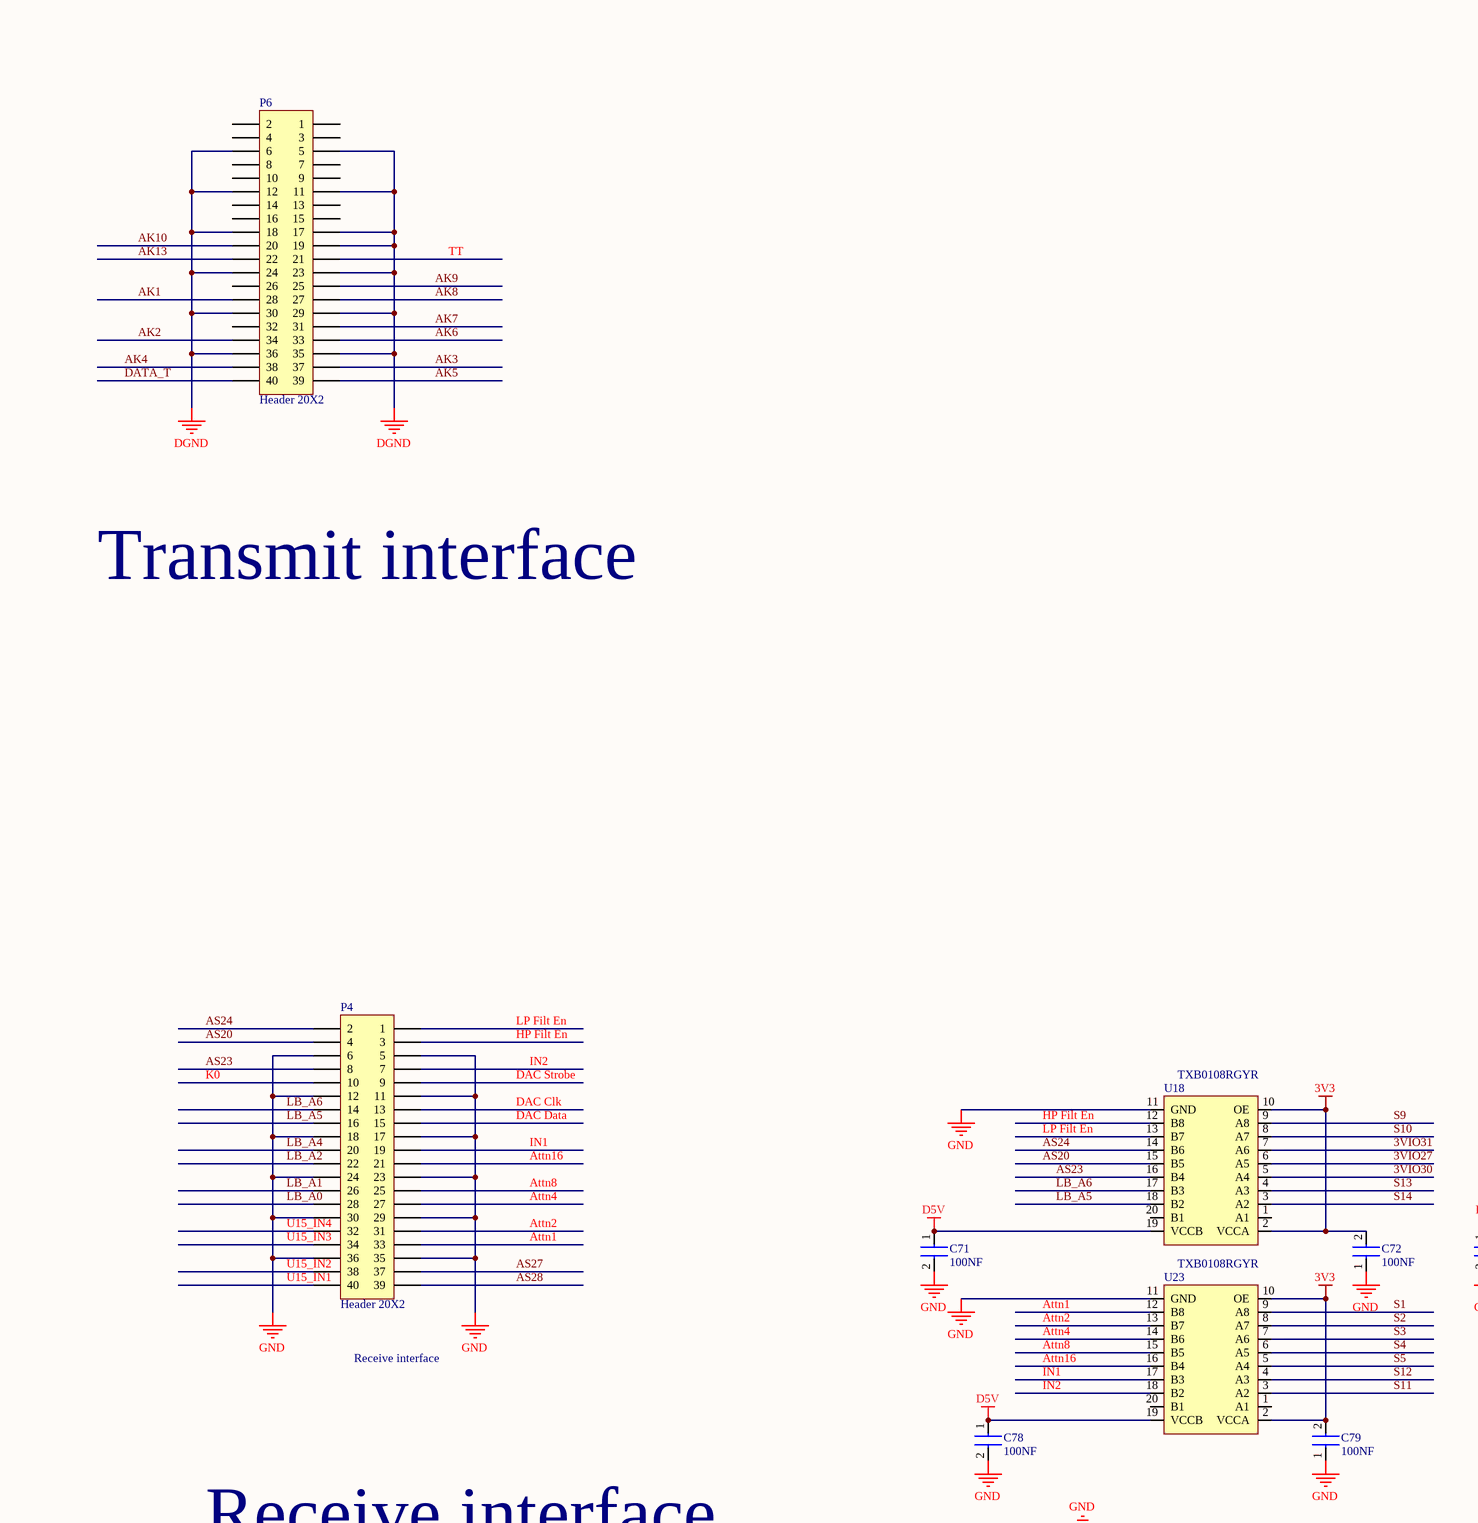
[diagram p0: MISC82191-3.SchDoc, top left]
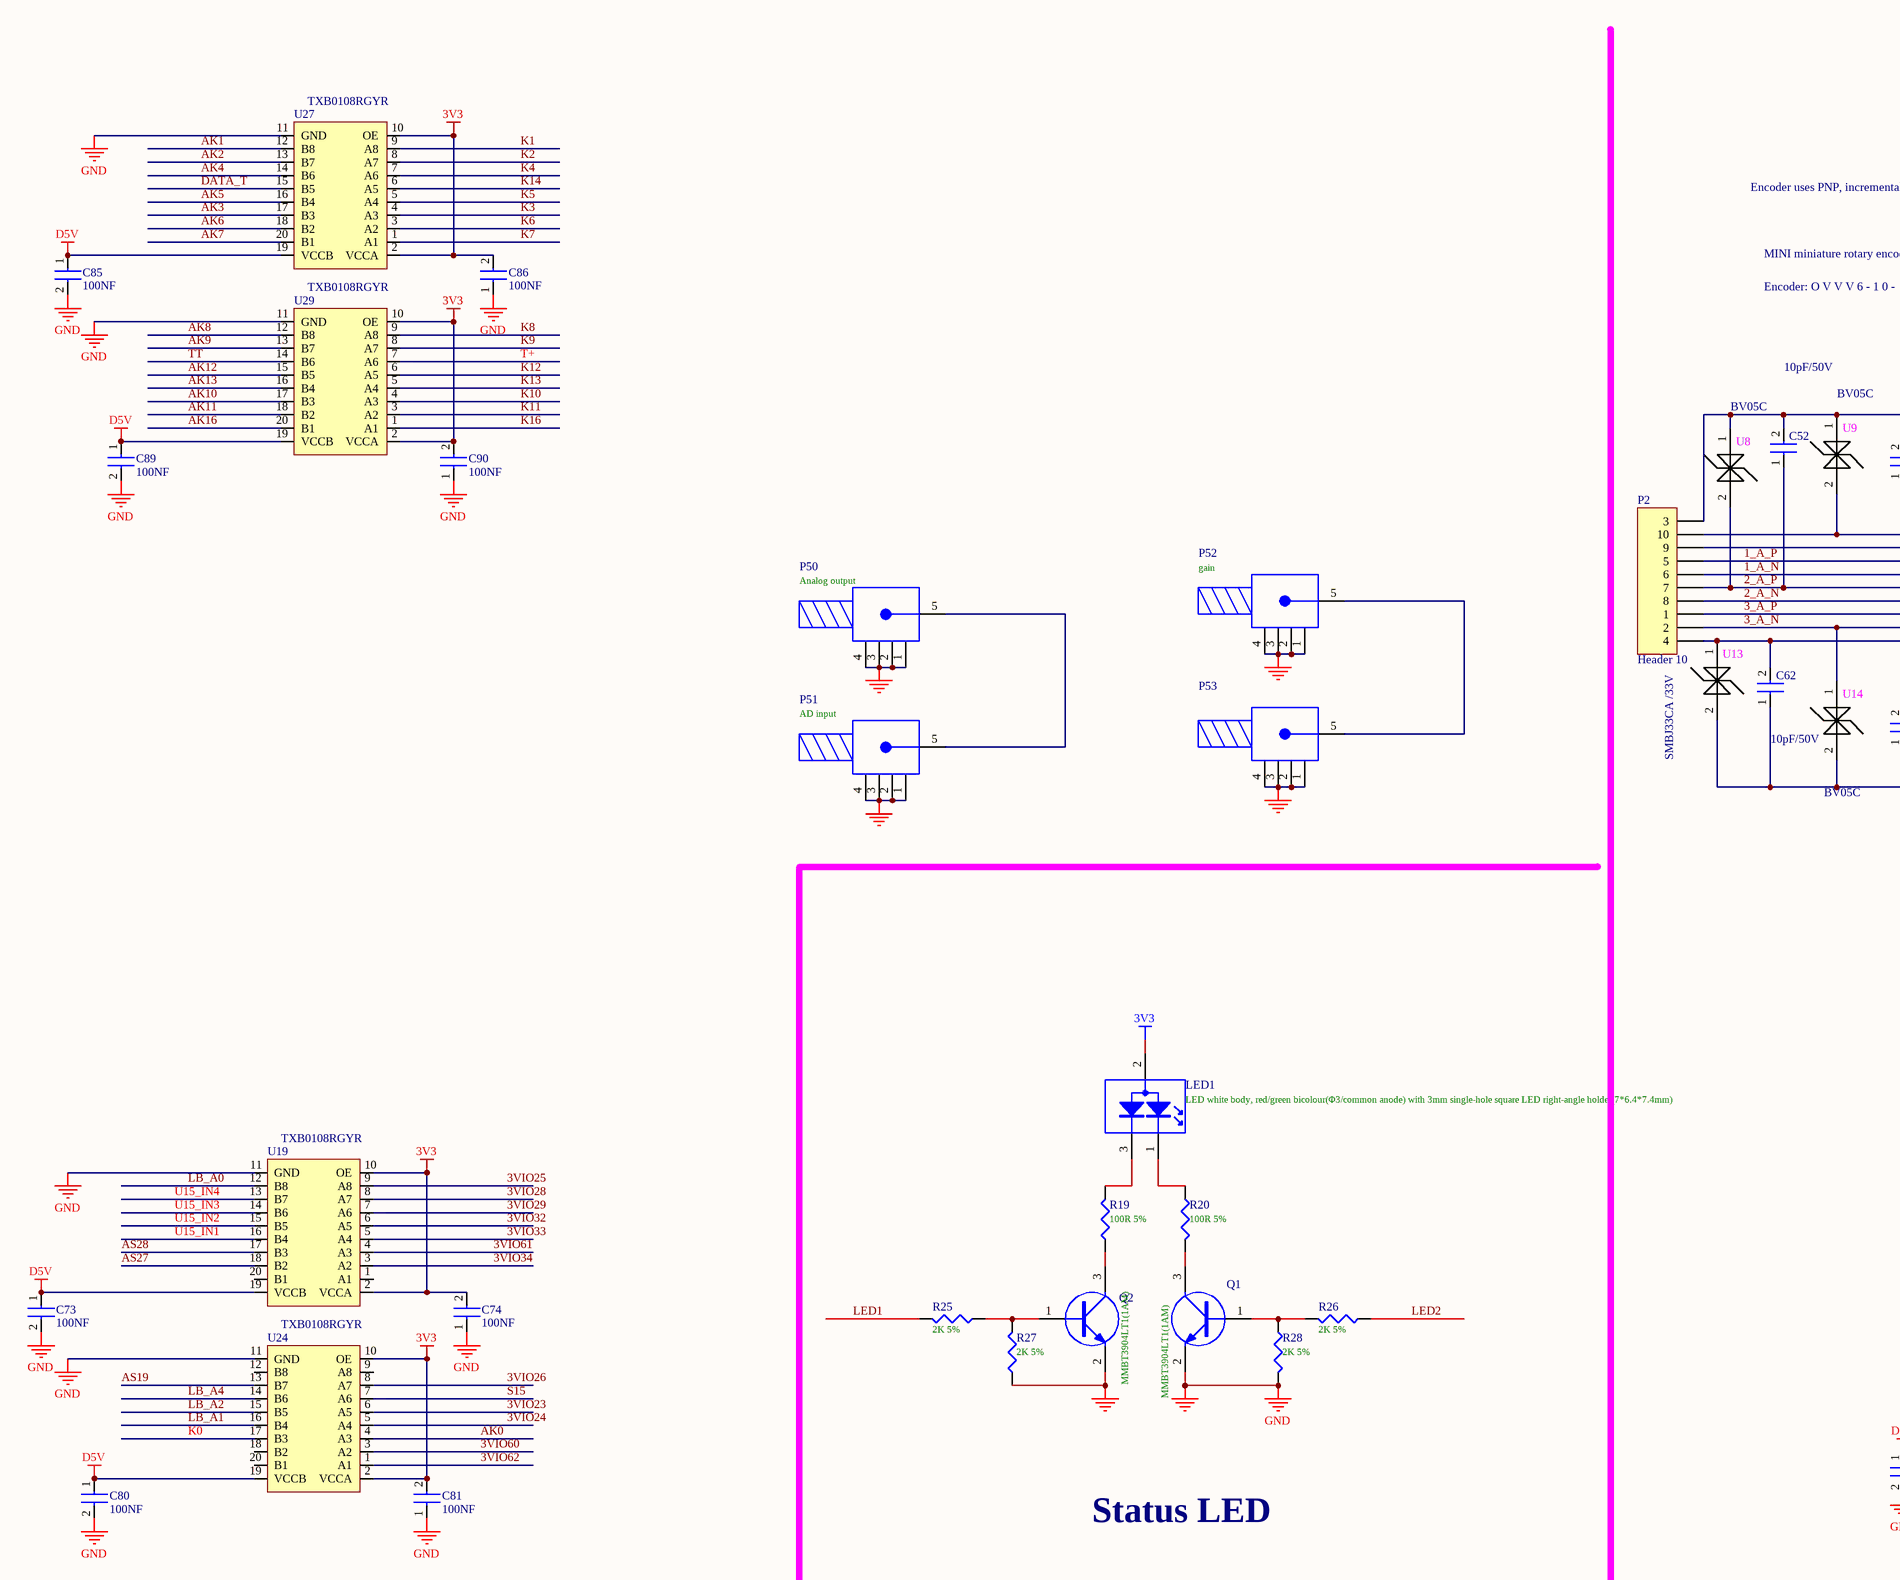
[diagram p1: MISC82191-3.SchDoc, top middle]
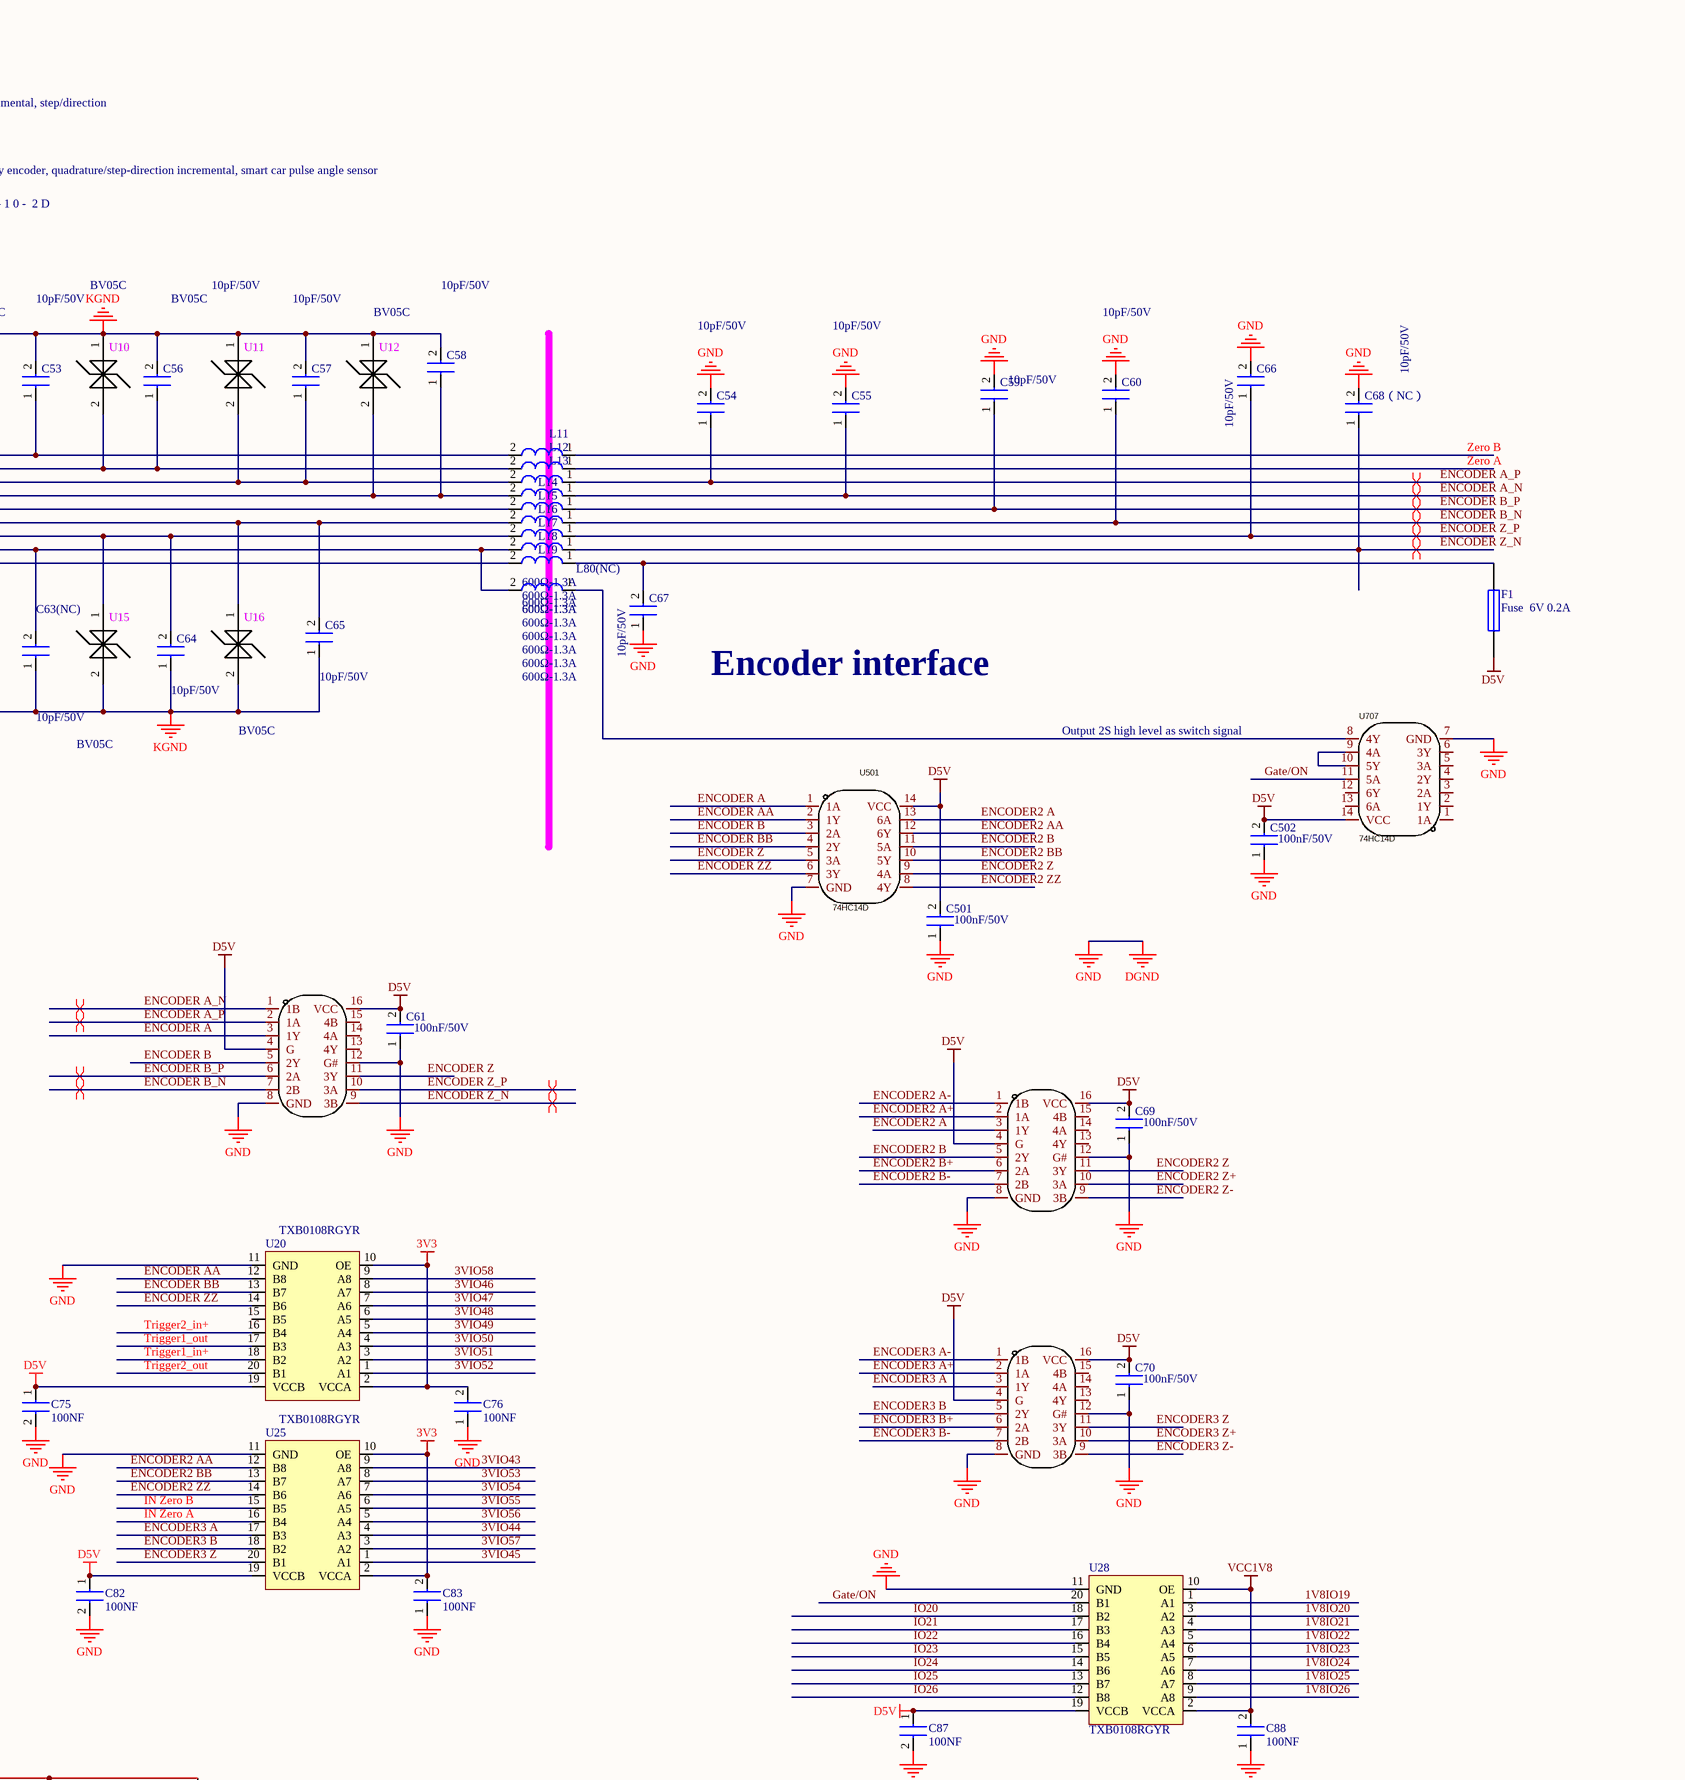
[diagram p2: MISC82191-3.SchDoc, top right]
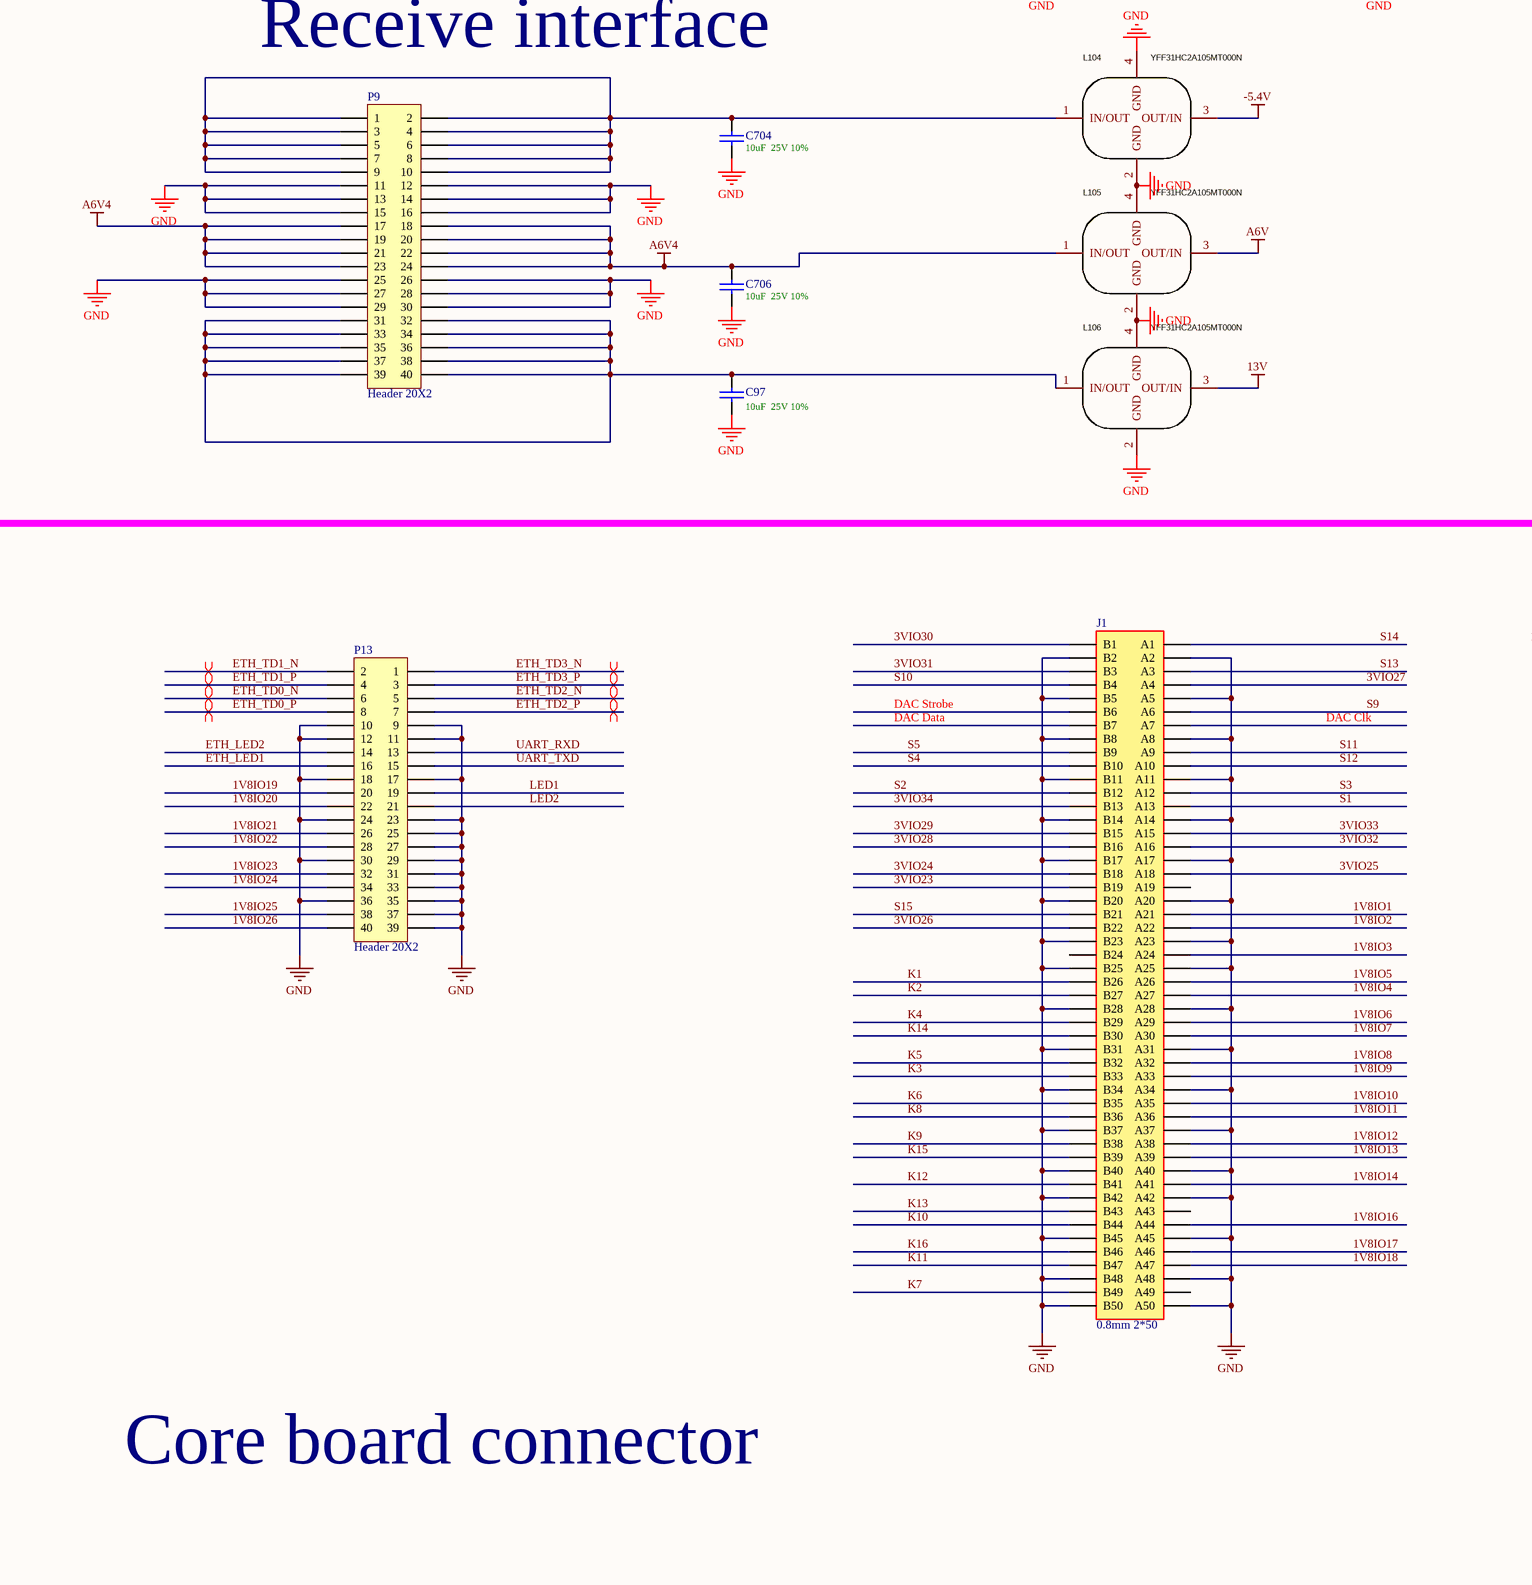
[diagram p3: MISC82191-3.SchDoc, bottom left]
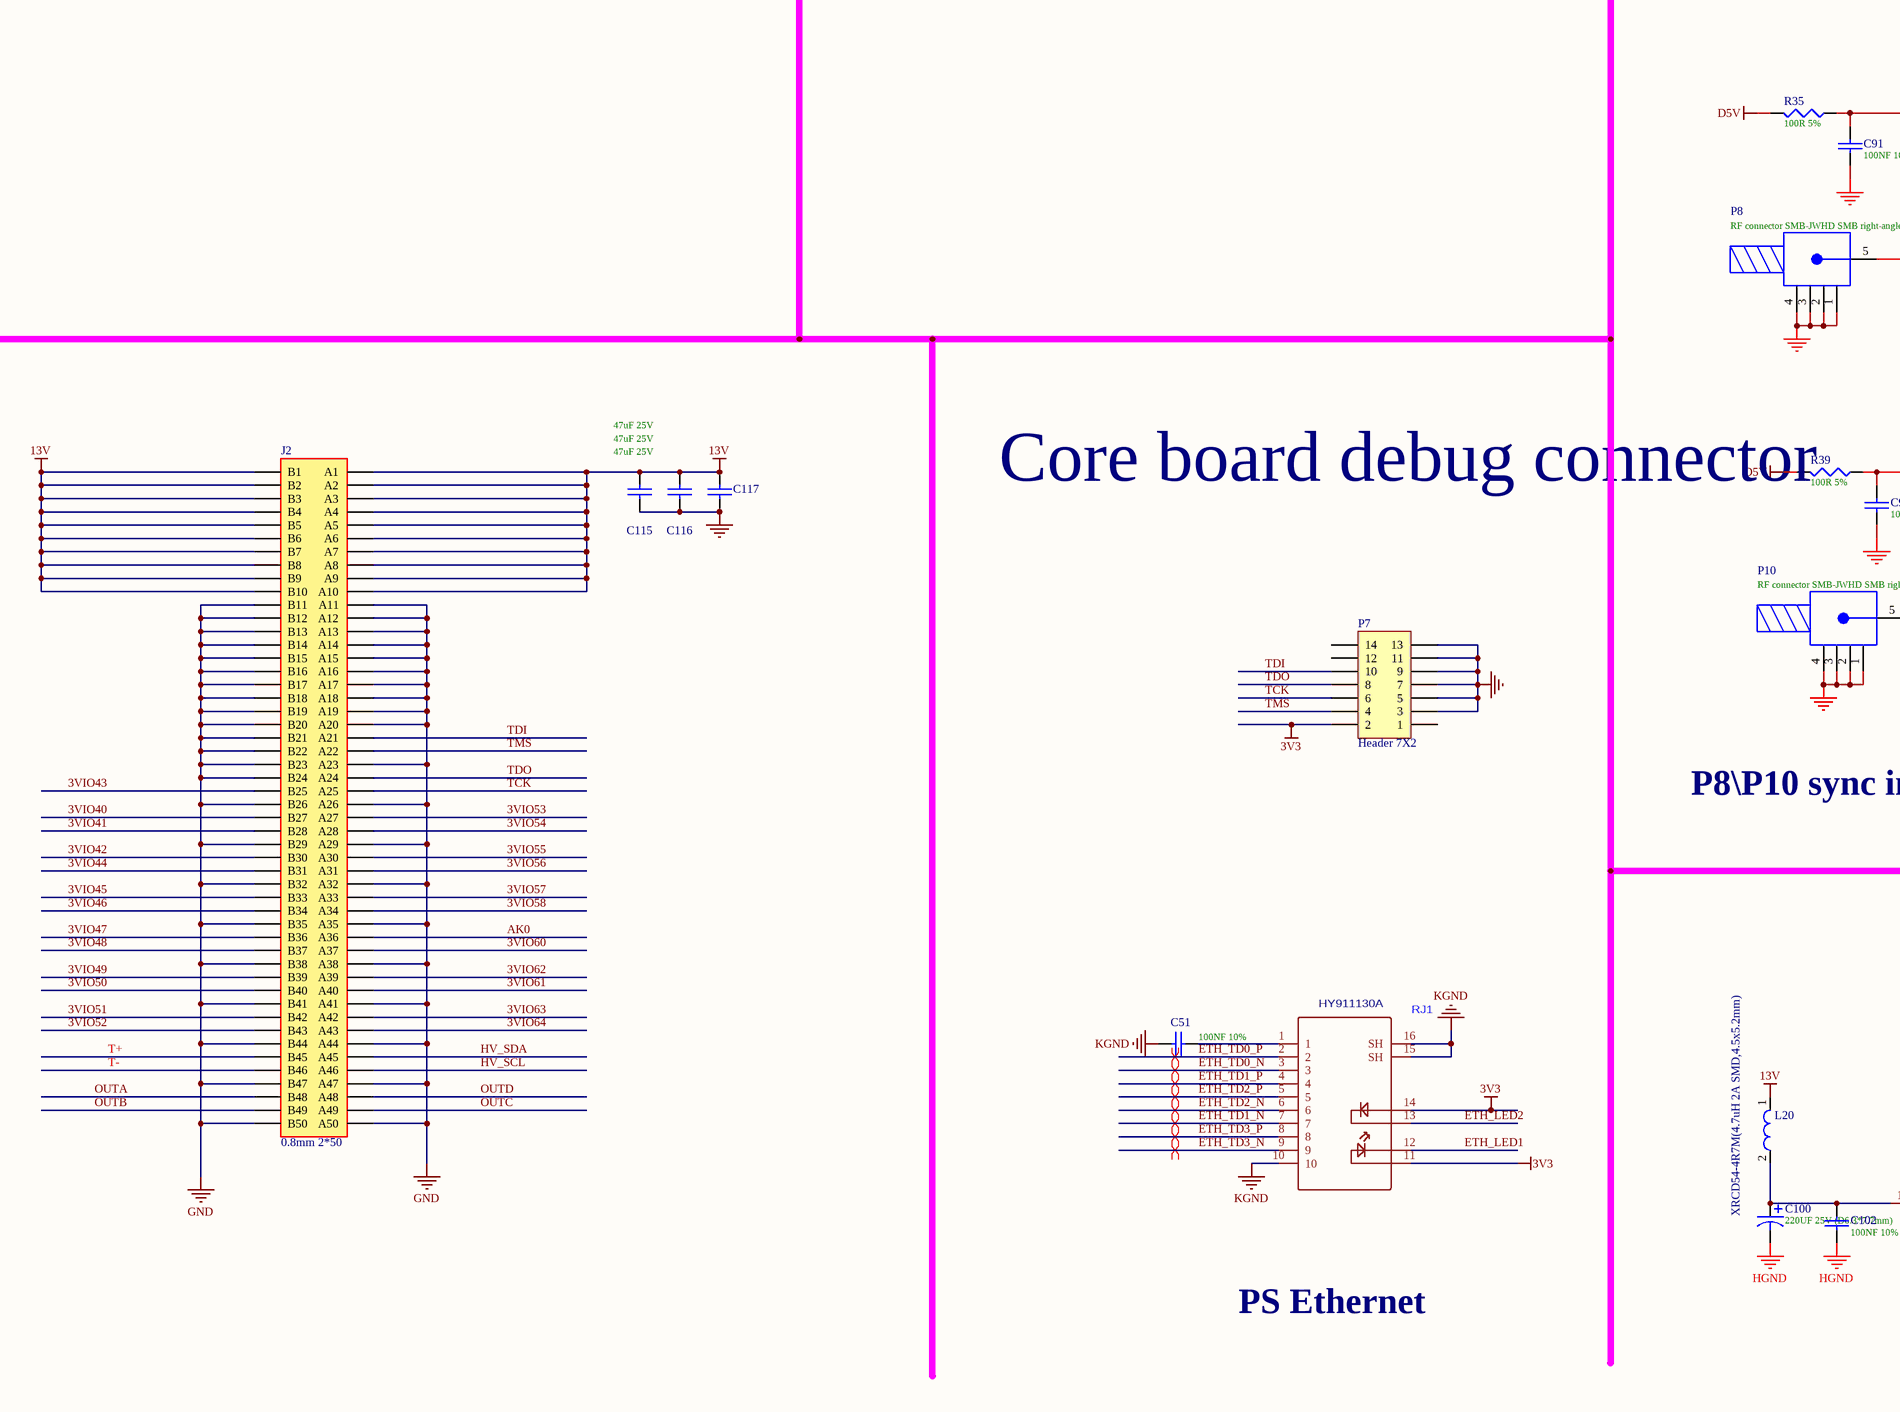
[diagram p4: MISC82191-3.SchDoc, bottom middle]
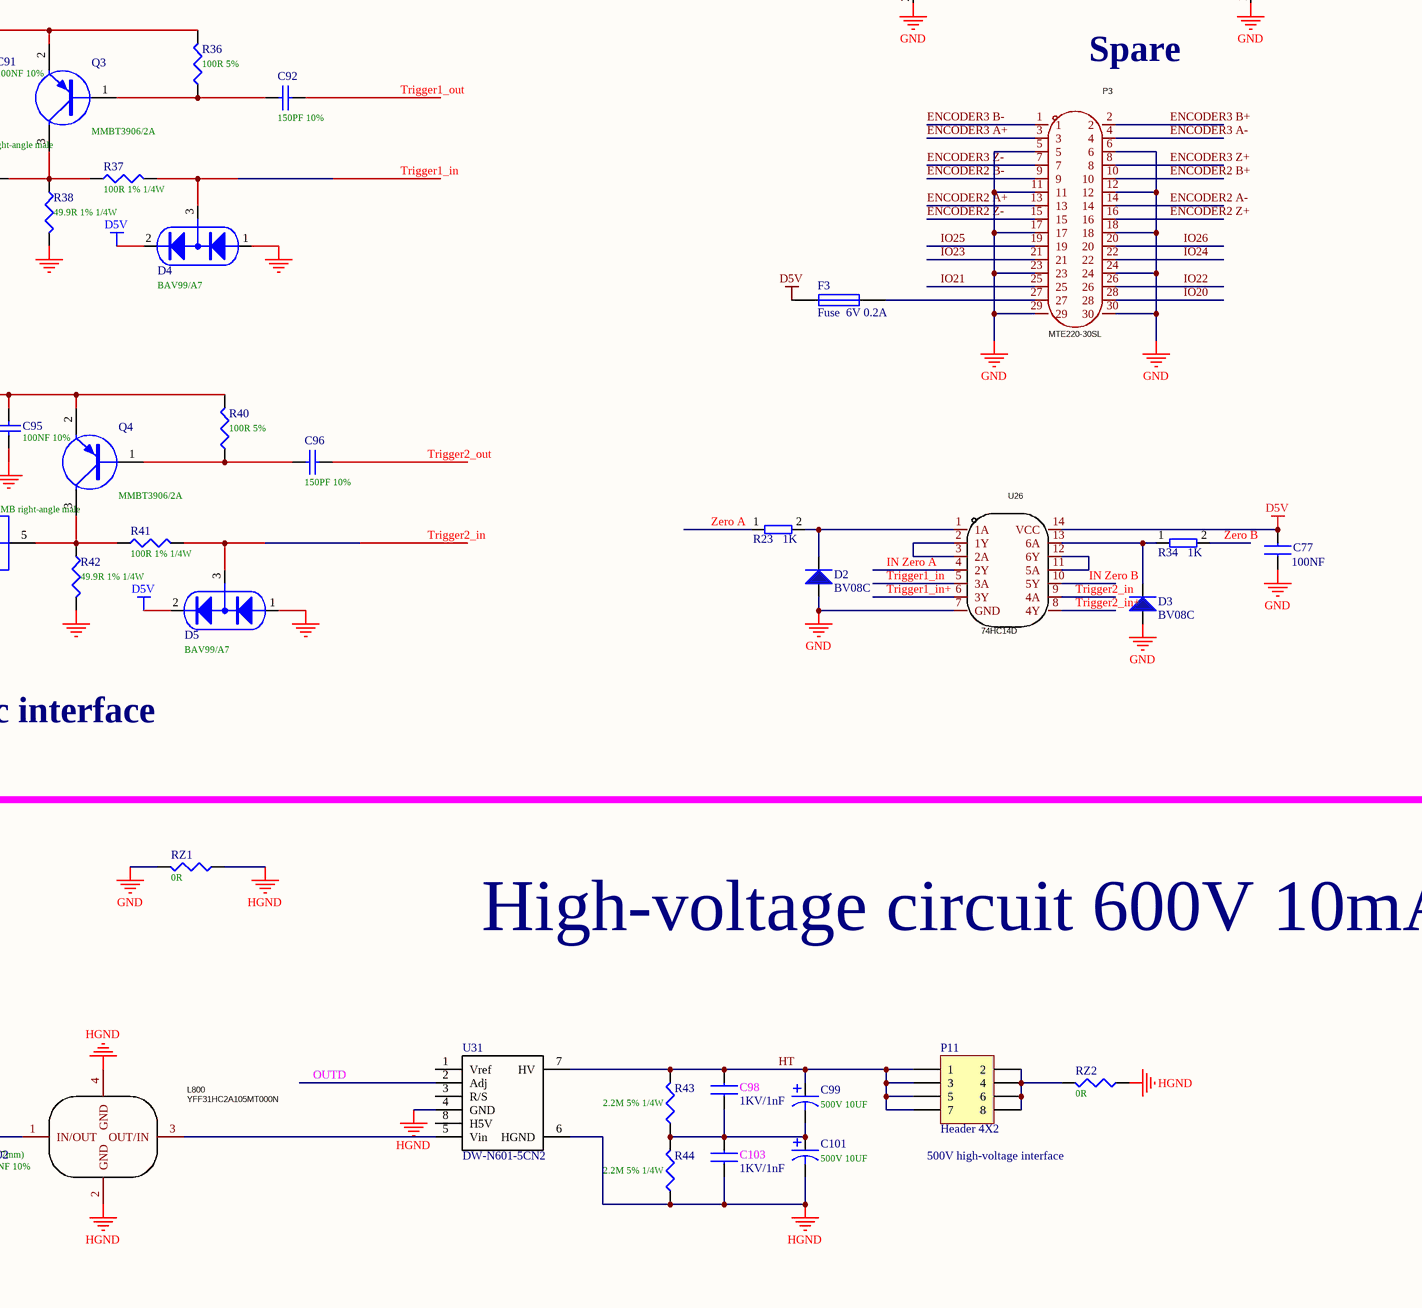
[diagram p5: MISC82191-3.SchDoc, bottom right]
# Altium project MISC82191-2.PrjPcb (part 1 of 4)
3 sheets, 238 parts. Net scope: global (net labels, ports and power ports of the same name join across sheets).
Board file: MISC82191.PcbDoc
Sheets:
  MISC82191-3.SchDoc
  MISC82191-5.SchDoc
  MISC82191-4.SchDoc